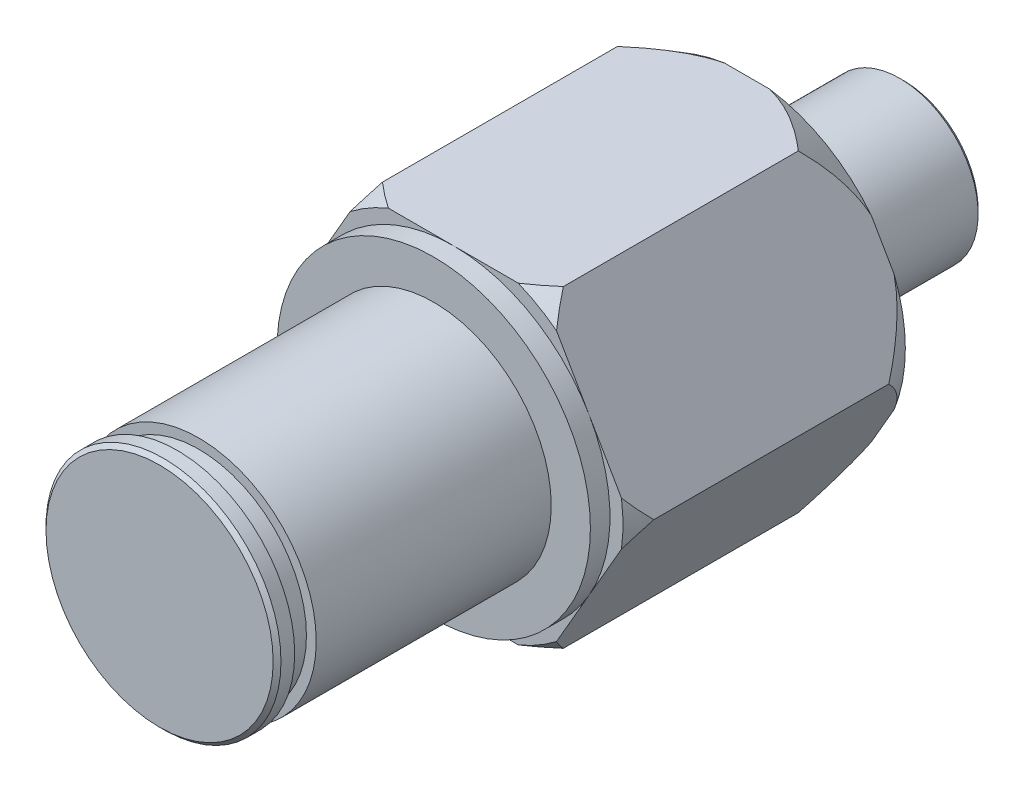
from build123d import *

# Parameters (mm, degrees)
SKETCH1_R           = 12.5
BOSS_EXTRUDE1_DEPTH = 30
SKETCH2_OUTSIDE_W   = 36.274
SKETCH2_OUTSIDE_H   = 36.274
CUT_EXTRUDE1_DEPTH  = 15
SKETCH3_OUTSIDE_W   = 36.274
SKETCH3_OUTSIDE_H   = 36.274
SKETCH3_OUTSIDE_R   = 8
CUT_EXTRUDE2_DEPTH  = 66.479004269
SKETCH4_R           = 4
BOSS_EXTRUDE2_DEPTH = 8
SKETCH5_OUTSIDE_W   = 29.512
SKETCH5_OUTSIDE_H   = 27.036
SKETCH5_OUTSIDE_R   = 3.25
CUT_EXTRUDE3_DEPTH  = 1.5
SKETCH6_OUTSIDE_W   = 29.512
SKETCH6_OUTSIDE_H   = 27.036
SKETCH6_OUTSIDE_R   = 6
CUT_EXTRUDE4_DEPTH  = 14
SKETCH8_OUTSIDE_W   = 29.512
SKETCH8_OUTSIDE_H   = 27.036
SKETCH8_OUTSIDE_R   = 5.5
CUT_EXTRUDE5_DEPTH  = 1.1
CHAMFER1_SIZE       = 0.2


with BuildPart() as part:
    # Sketch1 → Boss-Extrude1 (new body)
    with BuildSketch(Plane.XY):
        with Locations((0, 50)):
            Circle(SKETCH1_R)
    extrude(amount=BOSS_EXTRUDE1_DEPTH)

    # Sketch2 outside → Cut-Extrude1 (cut)
    with BuildSketch(Plane(origin=(0, 0, 0), x_dir=(-1, 0, 0), z_dir=(0, 0, -1))):
        with Locations((0, 50)):
            Rectangle(SKETCH2_OUTSIDE_W, SKETCH2_OUTSIDE_H)
        Polygon((-4.618802154, 42), (4.618802154, 42), (9.237604307, 50), (4.618802154, 58), (-4.618802154, 58), (-9.237604307, 50), align=None, mode=Mode.SUBTRACT)
    extrude(amount=-CUT_EXTRUDE1_DEPTH, mode=Mode.SUBTRACT)

    # Sketch3 outside → Cut-Extrude2 (cut, through all)
    with BuildSketch(Plane(origin=(0, 0, 15), x_dir=(-1, 0, 0), z_dir=(0, 0, -1))):
        with Locations((0, 50)):
            Rectangle(SKETCH3_OUTSIDE_W, SKETCH3_OUTSIDE_H)
        with Locations((0, 50)):
            Circle(SKETCH3_OUTSIDE_R, mode=Mode.SUBTRACT)
    extrude(amount=-CUT_EXTRUDE2_DEPTH, mode=Mode.SUBTRACT)

    # Sketch4 → Boss-Extrude2 (add)
    with BuildSketch(Plane(origin=(0, 0, 0), x_dir=(-1, 0, 0), z_dir=(0, 0, -1))):
        with Locations(Location((0, 50, 0), (0, 0, 180))):
            Circle(SKETCH4_R)
    extrude(amount=BOSS_EXTRUDE2_DEPTH)

    # Sketch5 outside → Cut-Extrude3 (cut)
    with BuildSketch(Plane(origin=(0, 0, 0), x_dir=(-1, 0, 0), z_dir=(0, 0, -1))):
        with Locations((0, 50)):
            Rectangle(SKETCH5_OUTSIDE_W, SKETCH5_OUTSIDE_H)
        with Locations((0, 50)):
            Circle(SKETCH5_OUTSIDE_R, mode=Mode.SUBTRACT)
    extrude(amount=CUT_EXTRUDE3_DEPTH, mode=Mode.SUBTRACT)

    # Sketch6 outside → Cut-Extrude4 (cut)
    with BuildSketch(Plane.XY.offset(30)):
        with Locations((0, 50)):
            Rectangle(SKETCH6_OUTSIDE_W, SKETCH6_OUTSIDE_H)
        with Locations((0, 50)):
            Circle(SKETCH6_OUTSIDE_R, mode=Mode.SUBTRACT)
    extrude(amount=-CUT_EXTRUDE4_DEPTH, mode=Mode.SUBTRACT)

    # Sketch8 outside → Cut-Extrude5 (cut)
    with BuildSketch(Plane.XY.offset(28)):
        with Locations((0, 50)):
            Rectangle(SKETCH8_OUTSIDE_W, SKETCH8_OUTSIDE_H)
        with Locations((0, 50)):
            Circle(SKETCH8_OUTSIDE_R, mode=Mode.SUBTRACT)
    extrude(amount=CUT_EXTRUDE5_DEPTH, mode=Mode.SUBTRACT)

    # Chamfer1
    chamfer1_edges = [part.edges().sort_by_distance(p)[0] for p in [
        (-4, 50, -8),
        (-6, 50, 30),
    ]]
    chamfer(chamfer1_edges, length=CHAMFER1_SIZE)

    # Sketch10 → Cut-Revolve1 (revolve, cut)
    with BuildSketch(Plane(origin=(0, 50, 0), x_dir=(1, 0, 0), z_dir=(0, 1, 0))):
        Polygon((-9.237604307, 0), (-9.237604307, -2), (-8.082903769, 0), align=None)
        Polygon((-9.237604307, -15), (-9.237604307, -14), (-8.660254038, -15), align=None)
    revolve(axis=Axis((0, 50, -8), (0, 0, 1)), mode=Mode.SUBTRACT)


solid = part.part
